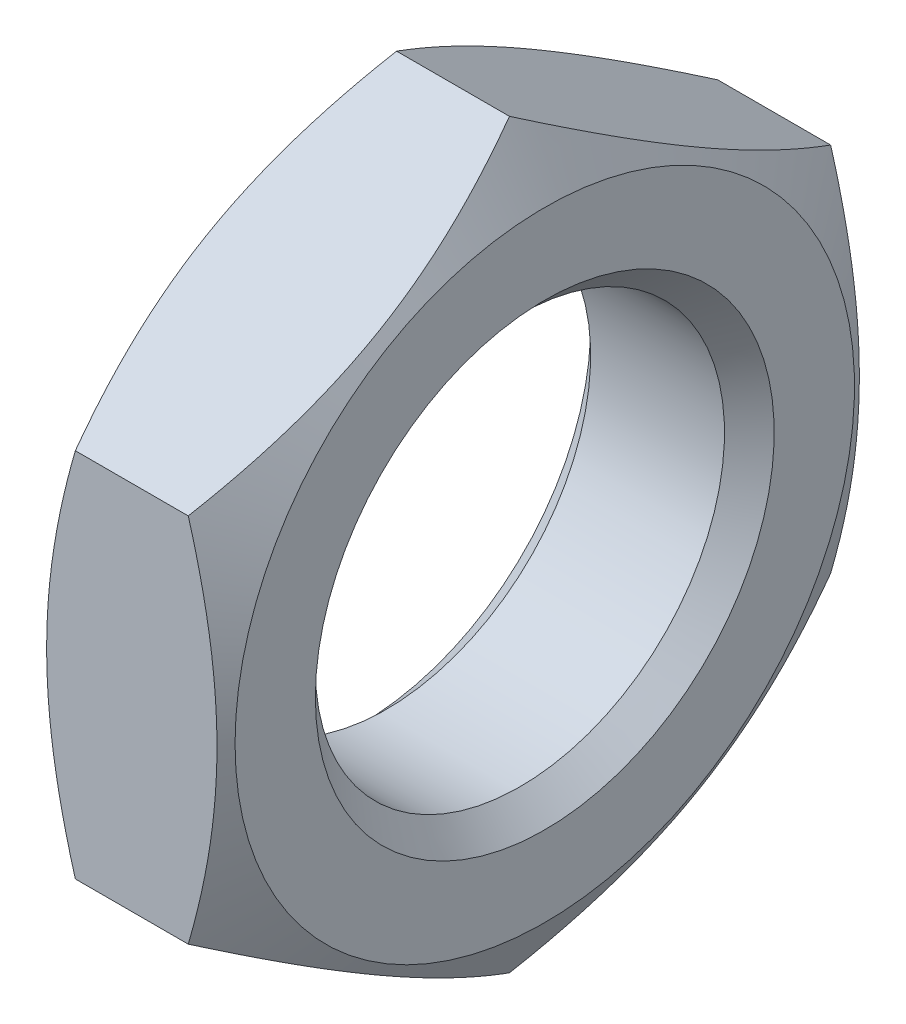
from build123d import *

# Parameters (mm, degrees)
EXTRUDE_1_DEPTH      = 2
EXTRUDE_1_DEPTH_BACK = 2


with BuildPart() as part:
    # 草图1 → 凸台-拉伸1 (new, two sides: drawn at the far end of the back side and taken through both)
    with BuildSketch(Plane(origin=(0, 0, 0), x_dir=(0, 0, -1), z_dir=(1, 0, 0)).offset(-EXTRUDE_1_DEPTH_BACK)):
        Polygon((-7, 4.041451884), (-7, -4.041451884), (0, -8.082903769), (7, -4.041451884), (7, 4.041451884), (0, 8.082903769), align=None)
    extrude(amount=EXTRUDE_1_DEPTH + EXTRUDE_1_DEPTH_BACK)

    # 草图2 → 切除-旋转1 (revolve, cut)
    with BuildSketch(Plane.XY, mode=Mode.PRIVATE) as cut_revolve_1_sk:
        Polygon((-2, 0), (-2, 5), (-1.4585, 4.4585), (1.4585, 4.4585), (2, 5), (2, 0), align=None)
    revolve(cut_revolve_1_sk.sketch.rotate(Axis((2, 0, 0), (-1, 0, 0)), 270), axis=Axis((2, 0, 0), (-1, 0, 0)), mode=Mode.SUBTRACT)

    # 草图3 → 切除-旋转2 (revolve, cut)
    with BuildSketch(Plane.XY, mode=Mode.PRIVATE) as cut_revolve_2_sk:
        Polygon((-7, 16.75), (-7, 1), (-2, 1), (-2, 6.75), (0, 10.214101615), (2, 6.75), (2, 1), (7, 1), (7, 16.75), align=None)
    revolve(cut_revolve_2_sk.sketch.rotate(Axis((50, 0, 0), (-1, 0, 0)), 270), axis=Axis((50, 0, 0), (-1, 0, 0)), mode=Mode.SUBTRACT)


solid = part.part
